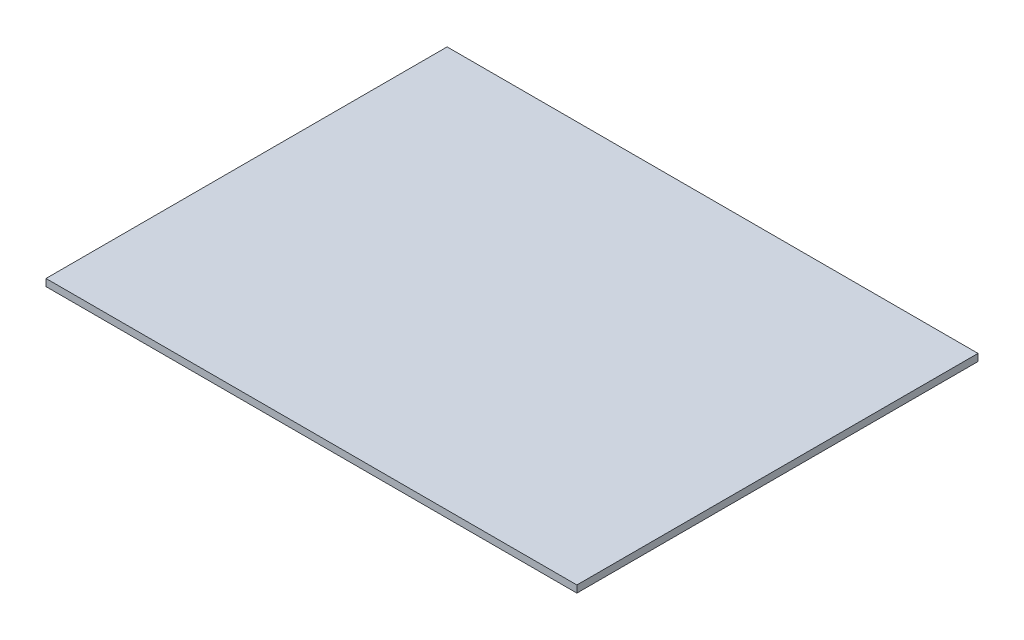
from build123d import *

# Parameters (mm, degrees)
SKETCH1_W           = 450
SKETCH1_H           = 340
BOSS_EXTRUDE1_DEPTH = 6


with BuildPart() as part:
    # Sketch1 → Boss-Extrude1 (new body)
    with BuildSketch(Plane(origin=(0, -5, 0), x_dir=(1, 0, 0), z_dir=(0, 1, 0))):
        with Locations((275, 230)):
            Rectangle(SKETCH1_W, SKETCH1_H)
    extrude(amount=-BOSS_EXTRUDE1_DEPTH)


solid = part.part
